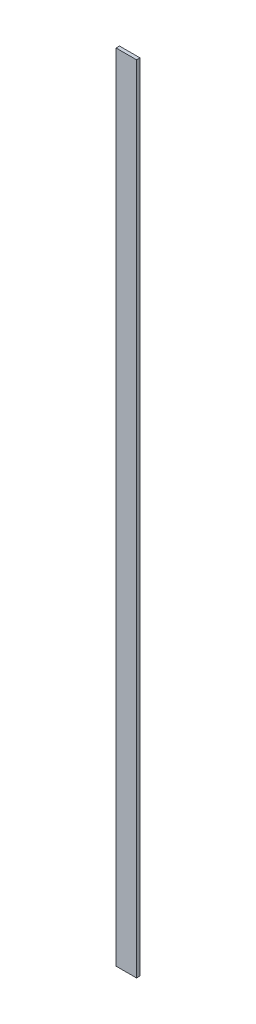
from build123d import *

# Parameters (mm, degrees)
SKETCH1_W           = 60
SKETCH1_H           = 2330
BOSS_EXTRUDE1_DEPTH = 10


with BuildPart() as part:
    # Sketch1 → Boss-Extrude1 (new body)
    with BuildSketch(Plane.XY):
        with Locations((30, 1165)):
            Rectangle(SKETCH1_W, SKETCH1_H)
    extrude(amount=BOSS_EXTRUDE1_DEPTH)


solid = part.part
